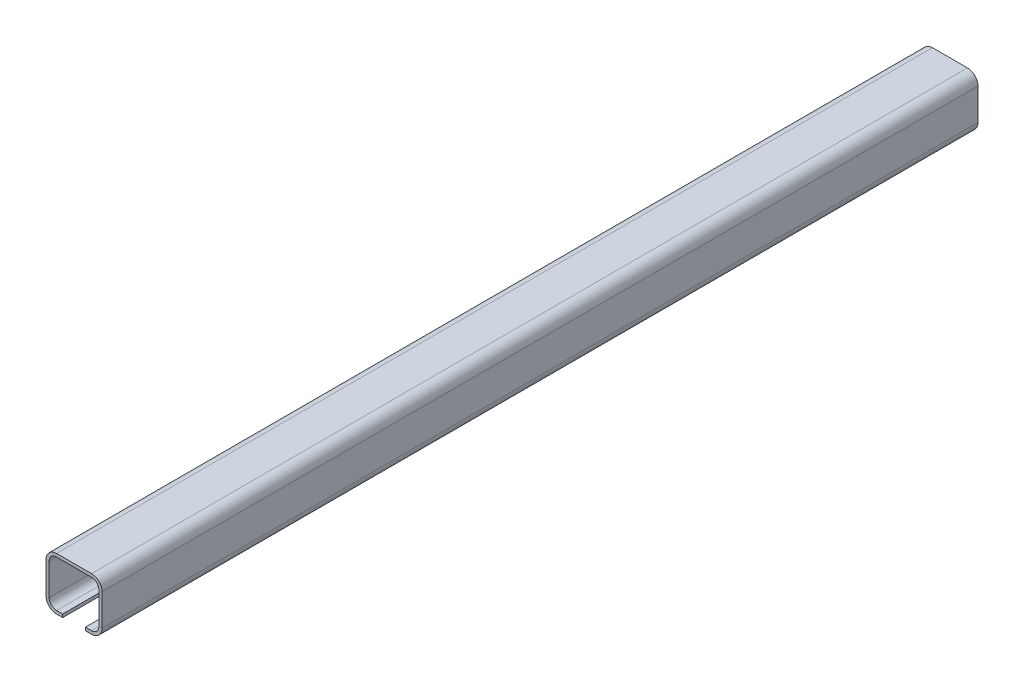
from build123d import *

# Parameters (mm, degrees)
BOSS_EXTRUDE1_DEPTH = 500


with BuildPart() as part:
    # Sketch1 → Boss-Extrude1 (new body)
    with BuildSketch(Plane.XY):
        with BuildLine():
            Line((-10, -13.2), (-6.5, -13.2))
            Line((-6.5, -13.2), (-6.5, -15))
            Line((-6.5, -15), (-10, -15))
            ThreePointArc((-10, -15), (-14.242640687, -13.242640687), (-16, -9))
            Line((-16, -9), (-16, 9))
            ThreePointArc((-16, 9), (-14.242640687, 13.242640687), (-10, 15))
            Line((-10, 15), (10, 15))
            ThreePointArc((10, 15), (14.242640687, 13.242640687), (16, 9))
            Line((16, 9), (16, -9))
            ThreePointArc((16, -9), (14.242640687, -13.242640687), (10, -15))
            Line((10, -15), (6.5, -15))
            Line((6.5, -15), (6.5, -13.2))
            Line((6.5, -13.2), (10, -13.2))
            ThreePointArc((10, -13.2), (12.969848481, -11.969848481), (14.2, -9))
            Line((14.2, -9), (14.2, 9))
            ThreePointArc((14.2, 9), (12.969848481, 11.969848481), (10, 13.2))
            Line((10, 13.2), (-10, 13.2))
            ThreePointArc((-10, 13.2), (-12.969848481, 11.969848481), (-14.2, 9))
            Line((-14.2, 9), (-14.2, -9))
            ThreePointArc((-14.2, -9), (-12.969848481, -11.969848481), (-10, -13.2))
        make_face()
    extrude(amount=BOSS_EXTRUDE1_DEPTH)


solid = part.part
